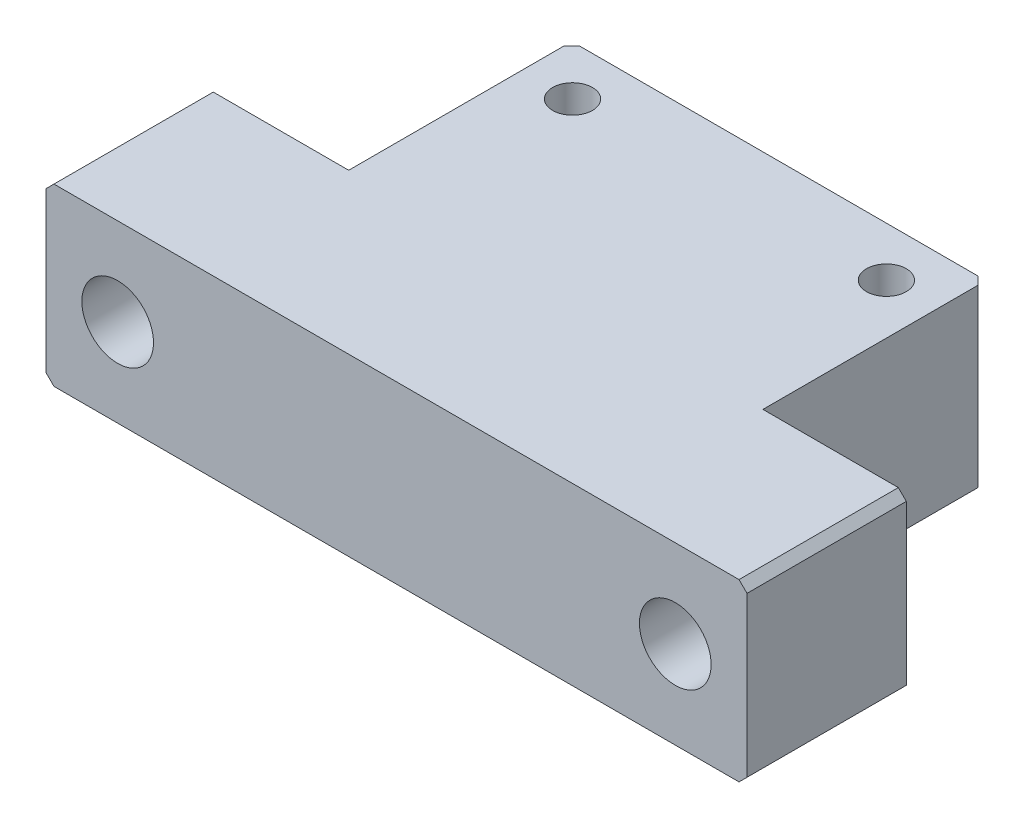
SolidWorks part; units mm, degrees
material "6061 合金"
ref_plane "Front Plane" through (0, 0, 0) normal (0, 0, 1) x (1, 0, 0)
ref_plane "Top Plane" through (0, 0, 0) normal (0, 1, 0) x (1, 0, 0)
ref_plane "Right Plane" through (0, 0, 0) normal (1, 0, 0) x (0, 0, -1)
sketch "Sketch1" plane through (0, 0, 0) normal (0, 0, 1) x (1, 0, 0)
  line L1 (-22, 5.5) -> (22, 5.5)
  line L2 (-22, 5.5) -> (-22, -5.5)
  line L3 (-22, -5.5) -> (22, -5.5)
  line L4 (22, 5.5) -> (22, -5.5)
  line L5 (-22, 5.5) -> (22, -5.5) construction
  line L6 (-22, -5.5) -> (22, 5.5) construction
  point P0 (0, 0)
  dimension "D1" = 44
  dimension "D2" = 11
extrude "Boss-Extrude1" add sketch "Sketch1" along normal blind 24
sketch "Sketch2" plane through (0, 5.5, 0) normal (0, 1, 0) x (1, 0, 0)
  line L1 (-22, -14) -> (-13, -14)
  line L2 (-22, -14) -> (-22, 0)
  line L3 (-22, 0) -> (-13, 0)
  line L4 (-13, -14) -> (-13, 0)
  line L5 (22, -14) -> (13, -14)
  line L6 (22, -14) -> (22, 0)
  line L7 (22, 0) -> (13, 0)
  line L8 (13, -14) -> (13, 0)
  line L9 (22, 0) -> (-22, 0) construction
  line L10 (22, -24) -> (22, 0) construction
  dimension "D1" = 14
  dimension "D2" = 26
extrude "Cut-Extrude1" cut sketch "Sketch2" against normal through all
hole_wizard "CBORE for M4 Hexagon socket head cap screws1" positions "Sketch3" profile "Sketch5" counterbore size "M4" standard "GB" end condition through all
sketch "Sketch3" plane through (0, 0, 14) normal (0, 0, -1) x (-1, 0, 0)
  line L0 (0, 0) -> (0, 3.5538) construction
  point P1 (-17.5, 0)
  point P3 (17.5, 0)
  dimension "D1" = 35
sketch "Sketch5" plane through (17.5, 0, 14) normal (1, 0, 0) x (0, 1, 0)
  line L0 (0, 0) -> (0, 10)
  line L1 (0, 10) -> (2.25, 10)
  line L3 (2.25, 10) -> (2.25, 4.6)
  line L4 (2.25, 4.6) -> (4, 4.6)
  line L5 (4, 4.6) -> (4, 0)
  line L7 (4, 0) -> (0, 0)
  line L11 (0, -6.35) -> (0, 107.95) construction
  dimension "通孔孔直径" = 4.5
  dimension "通孔孔深度" = 10
  dimension "柱形沉头孔直径" = 8
  dimension "柱形沉头孔深度" = 4.6
hole_wizard "M3 Tapped Hole1" positions "Sketch6" profile "Sketch7" tap size "M3" standard "GB" end condition through all
sketch "Sketch6" plane through (0, 5.5, 0) normal (0, 1, 0) x (1, 0, 0)
  line L0 (13, 0) -> (-13, 0) construction
  point P0 (9.85, -3.1)
  point P2 (-9.85, -3.1)
  dimension "D1" = 19.7
  dimension "D2" = 9.85
  dimension "D3" = 3.1
sketch "Sketch7" plane through (9.85, 5.5, 3.1) normal (1, 0, 0) x (0, 0, 1)
  line L0 (0, 0) -> (0, 11)
  line L1 (0, 11) -> (1.25, 11)
  line L2 (1.25, 11) -> (1.25, 0)
  line L5 (1.25, 0) -> (0, 0)
  line L11 (0, -6.35) -> (0, 107.95) construction
  dimension "通孔螺纹孔钻头直径" = 2.5
  dimension "通孔螺纹孔钻头深度" = 11
cosmetic thread "Cosmetic Thread1" parameters "D2"=3
cosmetic thread "Cosmetic Thread2" parameters "D2"=3
chamfer "Chamfer1" distance 0.5 angle 45 4 edges at (22, 5.5, 19) (22, -5.5, 19) (-22, 5.5, 19) (-22, -5.5, 19)
chamfer "Chamfer2" distance 0.5 angle 45 2 edges at (13, 0, 0) (-13, 0, 0)
